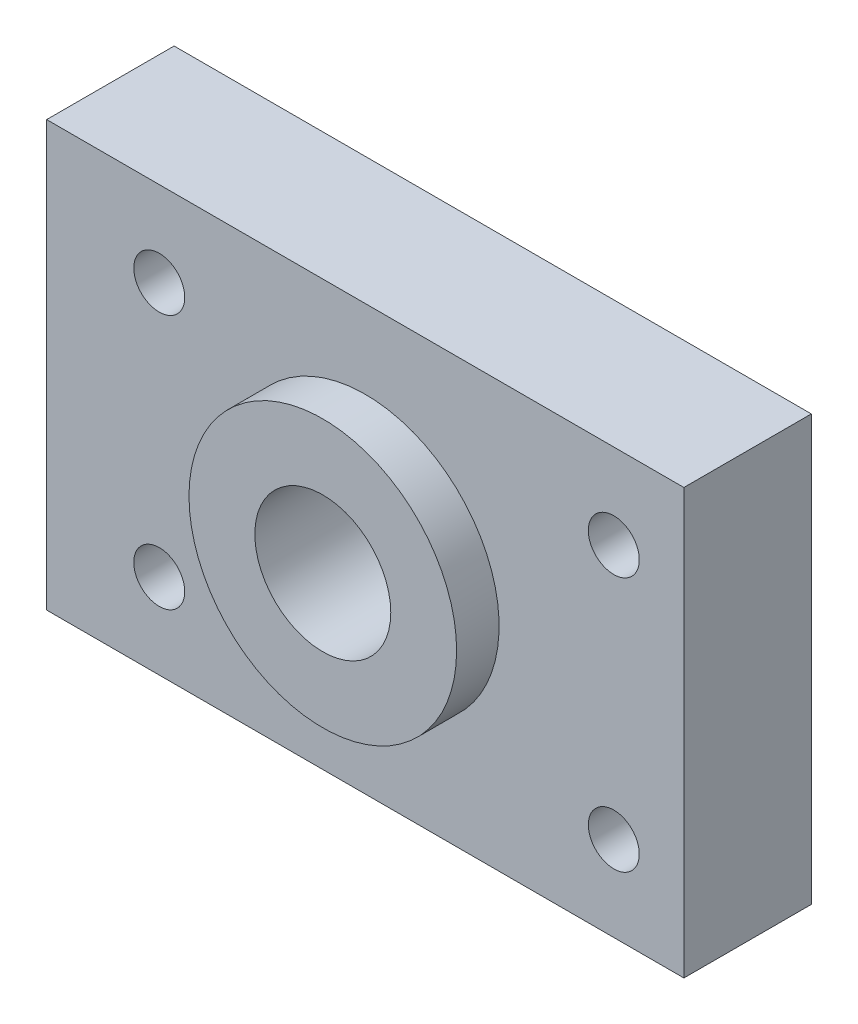
from build123d import *

# Parameters (mm, degrees)
SKETCH_1_W          = 150
SKETCH_1_H          = 100
EXTRUDE_1_DEPTH     = 30
SKETCH_2_R          = 31.5
SKETCH_2_R_2        = 16
EXTRUDE_2_DEPTH     = 10
SKETCH_3_R          = 16
CUT_EXTRUDE_1_DEPTH = 96
SKETCH_4_R          = 6
CUT_EXTRUDE_2_DEPTH = 99.615414617


with BuildPart() as part:
    # 草图1 → 凸台-拉伸1 (new body)
    with BuildSketch(Plane.XY):
        Rectangle(SKETCH_1_W, SKETCH_1_H)
    extrude(amount=EXTRUDE_1_DEPTH)

    # 草图2 → 凸台-拉伸2 (add)
    with BuildSketch(Plane.XY.offset(30)):
        with Locations(Location((0, 0, 0), (0, 0, 180))):
            Circle(SKETCH_2_R)
        Circle(SKETCH_2_R_2, mode=Mode.SUBTRACT)
    extrude(amount=EXTRUDE_2_DEPTH)

    # 草图3 → 切除-拉伸1 (cut, through all)
    with BuildSketch(Plane.XY.offset(30)):
        Circle(SKETCH_3_R)
    extrude(amount=-CUT_EXTRUDE_1_DEPTH, mode=Mode.SUBTRACT)

    # 草图4 → 切除-拉伸2 (cut, through all)
    with BuildSketch(Plane(origin=(0, 0, 0), x_dir=(-1, 0, 0), z_dir=(0, 0, -1))):
        with Locations((-58.5, 30)):
            Circle(SKETCH_4_R)
        with Locations((48.5, 30)):
            Circle(SKETCH_4_R)
        with Locations((48.5, -30)):
            Circle(SKETCH_4_R)
        with Locations((-58.5, -30)):
            Circle(SKETCH_4_R)
    extrude(amount=-CUT_EXTRUDE_2_DEPTH, mode=Mode.SUBTRACT)


solid = part.part
